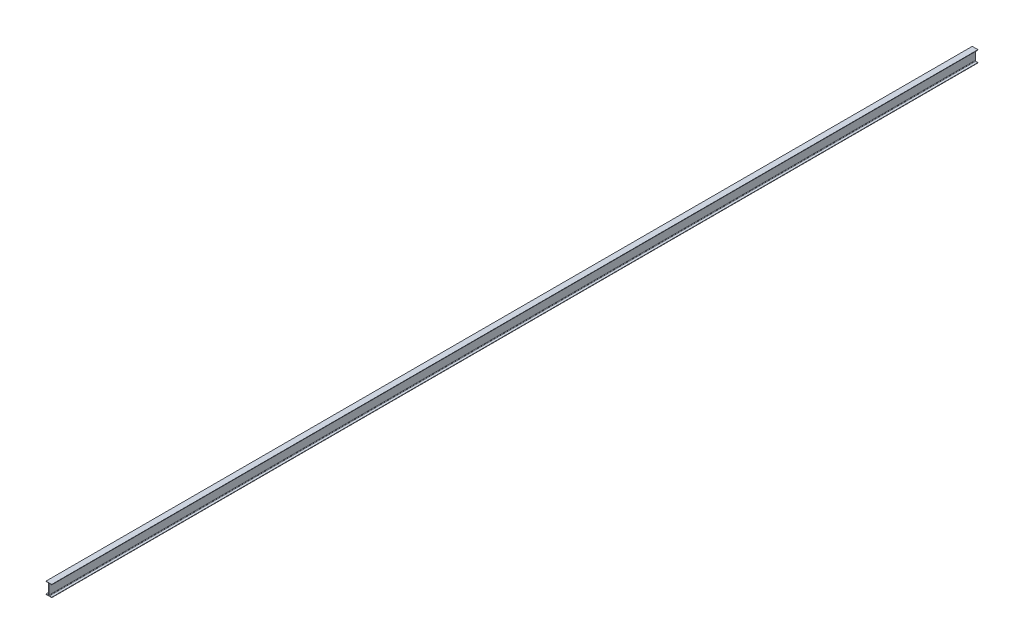
from build123d import *

# Parameters (mm, degrees)
BOSS_EXTRUDE1_DEPTH = 24174


with BuildPart() as part:
    # Sketch1 → Boss-Extrude1 (new body)
    with BuildSketch(Plane.XY):
        with BuildLine():
            Line((75, 0), (-75, 0))
            Line((-75, 0), (-75, 9))
            Line((-75, 9), (-16.25, 9))
            ThreePointArc((-16.25, 9), (-7.057611845, 12.807611845), (-3.25, 22))
            Line((-3.25, 22), (-3.25, 278))
            ThreePointArc((-3.25, 278), (-7.057611845, 287.192388155), (-16.25, 291))
            Line((-16.25, 291), (-75, 291))
            Line((-75, 291), (-75, 300))
            Line((-75, 300), (75, 300))
            Line((75, 300), (75, 291))
            Line((75, 291), (16.25, 291))
            ThreePointArc((16.25, 291), (7.057611845, 287.192388155), (3.25, 278))
            Line((3.25, 278), (3.25, 22))
            ThreePointArc((3.25, 22), (7.057611845, 12.807611845), (16.25, 9))
            Line((16.25, 9), (75, 9))
            Line((75, 9), (75, 0))
        make_face()
    extrude(amount=BOSS_EXTRUDE1_DEPTH)


solid = part.part
